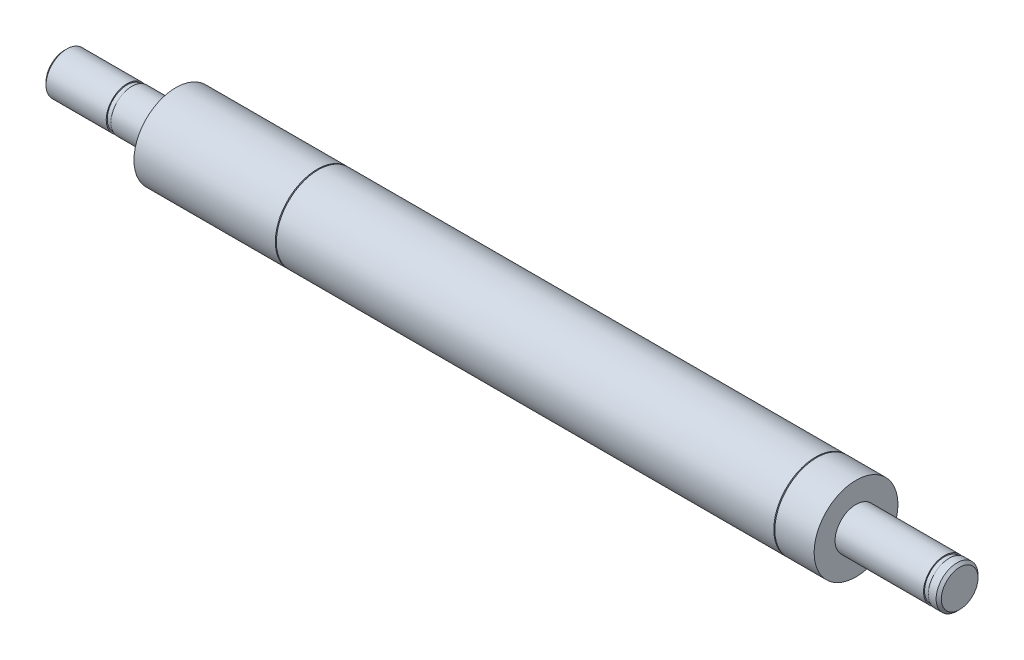
from build123d import *

# Parameters (mm, degrees)
SKETCH2_W     = 0.2
SKETCH2_H     = 1.6
SKETCH2_W_2   = 0.9
SKETCH2_H_2   = 0.2
CHAMFER1_SIZE = 0.5


with BuildPart() as part:
    # Sketch1 → Revolve1 (revolve)
    with BuildSketch(Plane(origin=(0, 0, 0), x_dir=(1, 0, 0), z_dir=(0, 1, 0))):
        Polygon((0, 0), (0, -4), (21.3, -4), (21.3, -8), (151.2, -8), (151.2, -4), (171, -4), (171, 0), align=None)
    revolve(axis=Axis((-12.256689328, 0, 0), (1, 0, 0)))

    # Sketch2 → Cut-Revolve1 (revolve, cut)
    with BuildSketch(Plane(origin=(0, 0, 0), x_dir=(1, 0, 0), z_dir=(0, 1, 0))):
        with Locations((48.4, -7.2)):
            Rectangle(SKETCH2_W, SKETCH2_H)
        with Locations((143.6, -7.2)):
            Rectangle(SKETCH2_W, SKETCH2_H)
        with Locations((168.55, -3.9)):
            Rectangle(SKETCH2_W_2, SKETCH2_H_2)
        with Locations((12.45, -3.9)):
            Rectangle(SKETCH2_W_2, SKETCH2_H_2)
    revolve(axis=Axis((-6.355227553, 0, 0), (1, 0, 0)), mode=Mode.SUBTRACT)

    # Chamfer1
    chamfer1_edges = [part.edges().sort_by_distance(p)[0] for p in [
        (171, 0, -4),
        (0, 0, -4),
    ]]
    chamfer(chamfer1_edges, length=CHAMFER1_SIZE)


solid = part.part
